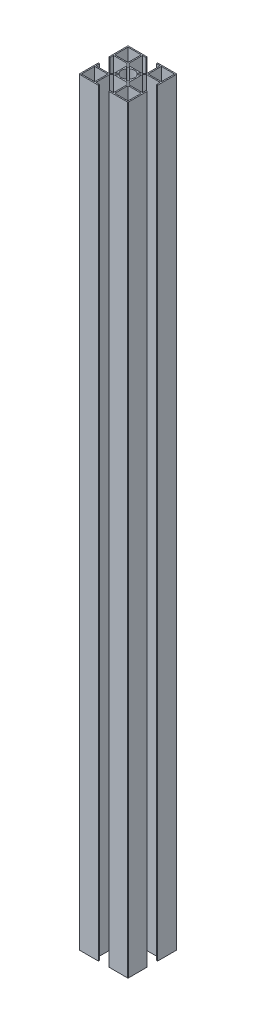
SolidWorks part; units mm, degrees
material "6061 Aluminium alloy"
ref_plane "Front" through (0, 0, 0) normal (0, 0, 1) x (1, 0, 0)
ref_plane "Top" through (0, 0, 0) normal (0, 1, 0) x (1, 0, 0)
ref_plane "Right" through (0, 0, 0) normal (1, 0, 0) x (0, 0, -1)
sketch "Sketch1" plane through (0, 0, 0) normal (0, 1, 0) x (1, 0, 0)
  line L0 (0, 0) -> (0, 20) construction
  line L1 (0, 0) -> (-20, 0) construction
  line L2 (-4.3, 20) -> (-19.5, 20)
  line L3 (-20, 19.5) -> (-20, 4.3)
  line L4 (-20, 4.3) -> (-19.05, 4.3)
  line L5 (-19.05, 4.3) -> (-19.05, 7.25)
  line L6 (-19.05, 7.25) -> (-7.9218, 7.25)
  line L7 (0, 0) -> (-4.3841, 4.3841) construction
  line L8 (-4.3, 20) -> (-4.3, 19.05)
  line L9 (-4.3, 19.05) -> (-7.25, 19.05)
  line L10 (-7.25, 19.05) -> (-7.25, 7.9218)
  line L11 (-7.25, 7.9218) -> (-5.5282, 6.2)
  line L12 (-8.2, 19.05) -> (-19.05, 19.05)
  line L13 (-19.05, 19.05) -> (-19.05, 8.2)
  line L14 (-19.05, 8.2) -> (-8.2, 8.2)
  line L15 (-7.9218, 7.25) -> (-6.2, 5.5282)
  line L16 (-8.2, 19.05) -> (-8.2, 8.2)
  line L17 (-5.5282, 6.2) -> (0, 6.2)
  line L18 (-6.2, 5.5282) -> (-6.2, 0)
  line L19 (-5.0912, 3.677) -> (-4.3875, 2.9732)
  line L20 (-3.677, 5.0912) -> (-2.9732, 4.3875)
  line L21 (0, 6.2) -> (0, 5.3)
  line L22 (-5.3, 0) -> (-6.2, 0)
  arc A0 (-4.3875, 2.9732) -> (-5.3, 0) centre (0, 0) ccw
  arc A1 (-19.5, 20) -> (-20, 19.5) centre (-19.5, 19.5) ccw
  circle A2 centre (0, 0) radius 7.2 construction
  arc A3 (-3.677, 5.0912) -> (-5.0912, 3.677) centre (-4.3841, 4.3841) ccw
  arc A4 (0, 5.3) -> (-2.9732, 4.3875) centre (0, 0) ccw
  dimension "D1" = 10.6
  dimension "D5" = 0.5
  dimension "D17" = 14.4
  dimension "D18" = 2
  dimension "D2" = 40
  dimension "D3" = 40
  dimension "D4" = 8.6
  dimension "D6" = 0.95
  dimension "D7" = 8.6
  dimension "D8" = 14.5
  dimension "D9" = 0.95
  dimension "D10" = 0.95
  dimension "D11" = 0.95
  dimension "D12" = 0.95
  dimension "D13" = 14.5
  dimension "D14" = 13.8
  dimension "D15" = 45
  dimension "D16" = 13.8
extrude "Boss-Extrude1" add sketch "Sketch1" along normal blind 620
mirror "Mirror1" about plane through (0, 0, 0) normal (1, 0, 0) of "Boss-Extrude1"
mirror "Mirror2" about plane through (0, 0, 0) normal (0, 0, 1) of "Mirror1", "Boss-Extrude1"
